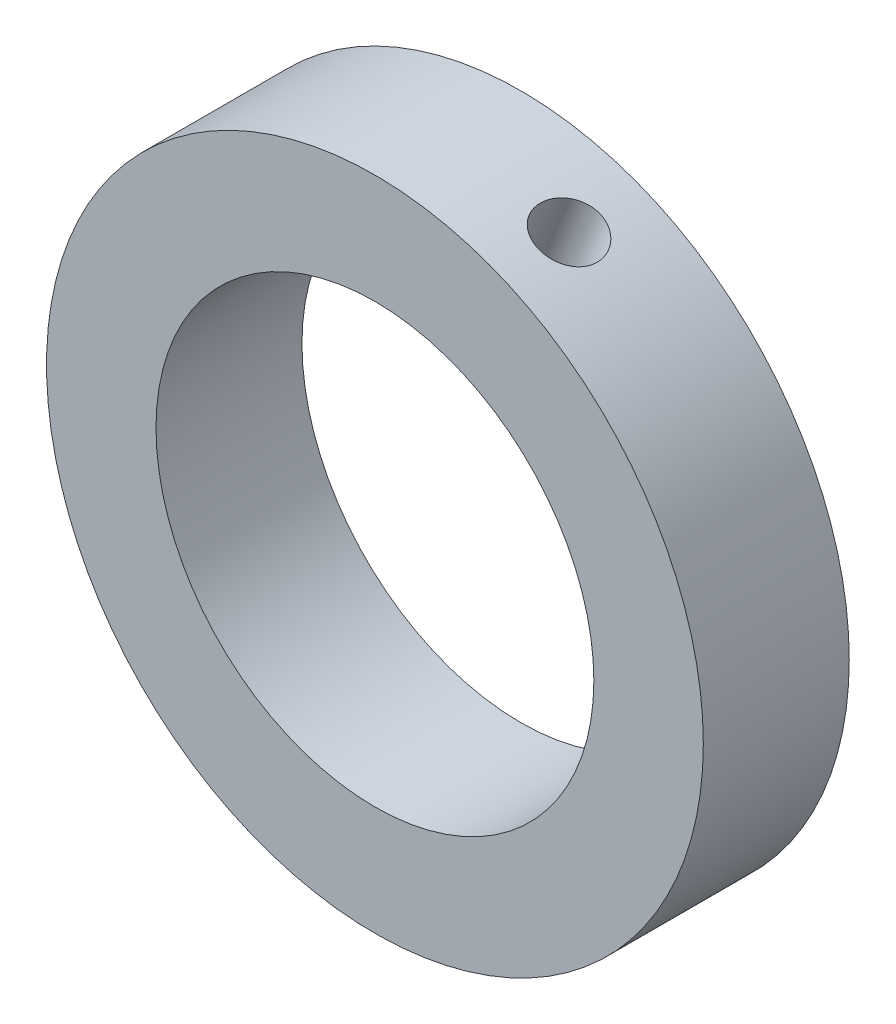
SolidWorks part; units mm, degrees
ref_plane "Front Plane" through (0, 0, 0) normal (0, 0, 1) x (1, 0, 0)
ref_plane "Top Plane" through (0, 0, 0) normal (0, 1, 0) x (1, 0, 0)
ref_plane "Right Plane" through (0, 0, 0) normal (1, 0, 0) x (0, 0, -1)
sketch "Sketch1" plane through (0, 0, 0) normal (0, 0, 1) x (1, 0, 0)
  circle A0 centre (0, 0) radius 15
  circle A1 centre (0, 0) radius 22.5
  dimension "D1" = 30
  dimension "D2" = 45
extrude "Boss-Extrude1" add sketch "Sketch1" along normal blind 10
hole_wizard "M5 Tapped Hole1" positions "3DSketch1" profile "Sketch2" tap size "M5" standard "GB"
sketch3d "3DSketch1"
  point P0 (8.3856, 20.879, 5.0691)
sketch "Sketch2" plane through (8.3856, 20.879, 5.0691) normal (0, 0, 1) x (-0.928, 0.3727, 0)
  line L0 (0, 0) -> (0, 7.5)
  line L1 (0, 7.5) -> (2.1, 7.5)
  line L2 (2.1, 7.5) -> (2.1, 0)
  line L5 (2.1, 0) -> (0, 0)
  line L11 (0, -6.35) -> (0, 107.95) construction
  dimension "通孔螺纹孔钻头直径" = 4.2
  dimension "通孔螺纹孔钻头深度" = 7.5
cosmetic thread "Hole thread1" parameters "D2"=5
